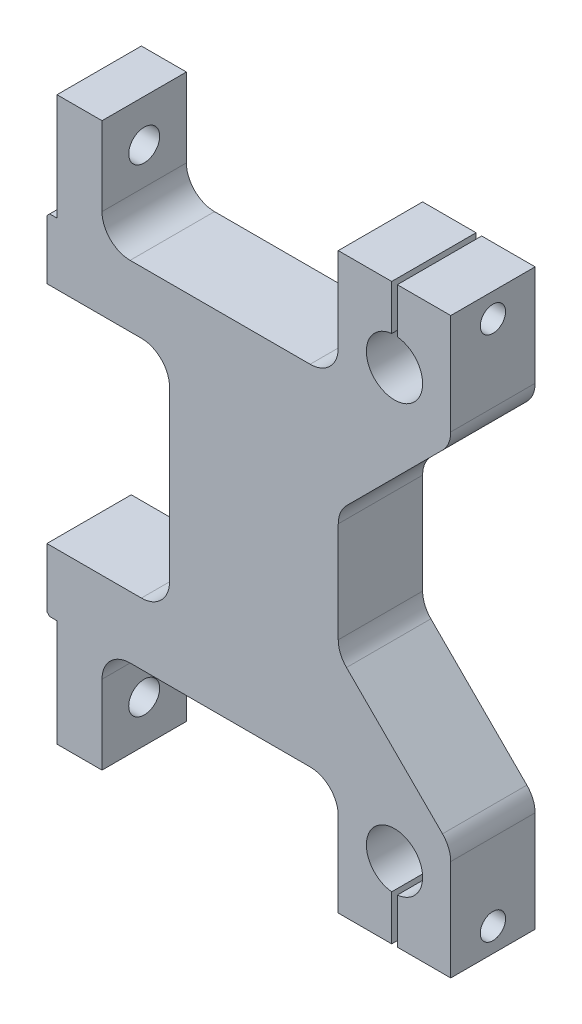
from build123d import *

# Parameters (mm, degrees)
BOSS_EXTRUDE1_DEPTH   = 40
SKETCH2_W             = 52
SKETCH2_H             = 20
CUT_EXTRUDE1_DEPTH    = 56
SKETCH3_R             = 5
CUT_EXTRUDE2_DEPTH    = 56
CHAMFER1_SIZE         = 20
SKETCH4_W             = 30
SKETCH4_H             = 11
BOSS_EXTRUDE2_DEPTH   = 15
SKETCH5_R             = 5
BOSS_EXTRUDE3_DEPTH   = 15
SKETCH6_W             = 45
SKETCH6_H             = 20
BOSS_EXTRUDE4_DEPTH   = 10
CUT_EXTRUDE3_REACH    = 134.714
SKETCH8_W             = 47.061475946
SKETCH8_H             = 40
SKETCH9_W             = 45
SKETCH9_H             = 19
BOSS_EXTRUDE5_DEPTH   = 8
SKETCH11_R            = 2.75
CUT_EXTRUDE4_DEPTH    = 37
SKETCH12_W            = 30
SKETCH12_H            = 100
CUT_EXTRUDE5_DEPTH    = 112
SKETCH13_W            = 0.2
SKETCH13_H            = 62
CUT_EXTRUDE6_DEPTH    = 112
CHAMFER2_SIZE         = 0.5
SKETCH14_W            = 1
SKETCH14_H            = 9.442903458
CUT_EXTRUDE7_DEPTH    = 29
SKETCH15_R            = 2.25
CUT_EXTRUDE8_DEPTH    = 9.5
M4_TAPPED_HOLE1_D     = 3.3
M4_TAPPED_HOLE1_DEPTH = 9.5
M4_TAPPED_HOLE2_D     = 3.3
M4_TAPPED_HOLE2_DEPTH = 9.5
FILLET1_R             = 5


with BuildPart() as part:
    # Sketch1 → Boss-Extrude1 (new body)
    with BuildSketch(Plane(origin=(0, 0, 0), x_dir=(1, 0, 0), z_dir=(0, 1, 0))):
        Polygon((0, 0), (72, 0), (72, 15), (10, 15), (10, 45), (0, 45), align=None)
    extrude(amount=BOSS_EXTRUDE1_DEPTH)

    # Sketch2 → Cut-Extrude1 (cut)
    with BuildSketch(Plane.XY):
        with Locations((26, 10)):
            Rectangle(SKETCH2_W, SKETCH2_H)
    extrude(amount=-CUT_EXTRUDE1_DEPTH, mode=Mode.SUBTRACT)

    # Sketch3 → Cut-Extrude2 (cut)
    with BuildSketch(Plane.XY):
        with Locations((62, 13)):
            Circle(SKETCH3_R)
    extrude(amount=-CUT_EXTRUDE2_DEPTH, mode=Mode.SUBTRACT)

    # Chamfer1
    chamfer1_edges = [part.edges().sort_by_distance(p)[0] for p in [
        (72, 40, -7.5),
    ]]
    chamfer(chamfer1_edges, length=CHAMFER1_SIZE)

    # Sketch4 → Boss-Extrude2 (add)
    with BuildSketch(Plane.XY):
        with Locations((37, 45.5)):
            Rectangle(SKETCH4_W, SKETCH4_H)
    extrude(amount=-BOSS_EXTRUDE2_DEPTH)

    # Sketch5 → Boss-Extrude3 (add)
    with BuildSketch(Plane.XY):
        Polygon((22, 51), (52, 51), (52, 62), (72, 82), (72, 102), (52, 102), (52, 82), (0, 82), (0, 62), (22, 62), align=None)
        with Locations((62, 89)):
            Circle(SKETCH5_R, mode=Mode.SUBTRACT)
    extrude(amount=-BOSS_EXTRUDE3_DEPTH)

    # Sketch6 → Boss-Extrude4 (add)
    with BuildSketch(Plane.ZY):
        with Locations((-22.5, 30)):
            Rectangle(SKETCH6_W, SKETCH6_H)
        with Locations((-22.5, 72)):
            Rectangle(SKETCH6_W, SKETCH6_H)
    extrude(amount=-BOSS_EXTRUDE4_DEPTH)

    # Cut-Extrude3: up to this face of the body (flat: up to its plane)
    cut_extrude3_end = Plane(part.part.faces().sort_by_distance((22, 51, -7.5))[0])
    # Sketch8 → Cut-Extrude3 (cut, up to the picked face)
    with BuildSketch(Plane.ZY, mode=Mode.PRIVATE) as cut_extrude3_sk1:
        with Locations((-21.469262027, 51)):
            Rectangle(SKETCH8_W, SKETCH8_H)
    cut_extrude3_tool1 = split(extrude(cut_extrude3_sk1.sketch, amount=-CUT_EXTRUDE3_REACH, mode=Mode.PRIVATE), bisect_by=cut_extrude3_end, keep=Keep.BOTH, mode=Mode.PRIVATE)
    add(cut_extrude3_tool1.solids().sort_by(Axis((0, 51, -21.469262), (1, 0, 0)))[0], mode=Mode.SUBTRACT)

    # Sketch9 → Boss-Extrude5 (add)
    with BuildSketch(Plane(origin=(10, 0, 0), x_dir=(0, 0, -1), z_dir=(1, 0, 0))):
        with Locations((22.5, 91.5)):
            Rectangle(SKETCH9_W, SKETCH9_H)
        with Locations((22.5, 10.5)):
            Rectangle(SKETCH9_W, SKETCH9_H)
    extrude(amount=-BOSS_EXTRUDE5_DEPTH)

    # Sketch11 → Cut-Extrude4 (cut)
    with BuildSketch(Plane(origin=(10, 0, 0), x_dir=(0, 0, -1), z_dir=(1, 0, 0))):
        with Locations((7.5, 93.5)):
            Circle(SKETCH11_R)
        with Locations(Location((7.5, 8.5, 0), (0, 0, 180))):
            Circle(SKETCH11_R)
    extrude(amount=-CUT_EXTRUDE4_DEPTH, mode=Mode.SUBTRACT)

    # Sketch12 → Cut-Extrude5 (cut)
    with BuildSketch(Plane(origin=(72, 0, 0), x_dir=(0, 0, -1), z_dir=(1, 0, 0))):
        with Locations((30, 51)):
            Rectangle(SKETCH12_W, SKETCH12_H)
    extrude(amount=-CUT_EXTRUDE5_DEPTH, mode=Mode.SUBTRACT)

    # Sketch13 → Cut-Extrude6 (cut)
    with BuildSketch(Plane.XY):
        with Locations((0.1, 51)):
            Rectangle(SKETCH13_W, SKETCH13_H)
    extrude(amount=-CUT_EXTRUDE6_DEPTH, mode=Mode.SUBTRACT)

    # Chamfer2
    chamfer2_edges = [part.edges().sort_by_distance(p)[0] for p in [
        (0.2, 20, -7.5),
        (0.2, 82, -7.5),
    ]]
    chamfer(chamfer2_edges, length=CHAMFER2_SIZE)

    # Sketch14 → Cut-Extrude7 (cut)
    with BuildSketch(Plane.XY):
        with Locations((62, 4.721451729)):
            Rectangle(SKETCH14_W, SKETCH14_H)
        with Locations((62, 97.278548271)):
            Rectangle(SKETCH14_W, SKETCH14_H)
    extrude(amount=-CUT_EXTRUDE7_DEPTH, mode=Mode.SUBTRACT)

    # Sketch15 → Cut-Extrude8 (cut)
    with BuildSketch(Plane(origin=(72, 0, 0), x_dir=(0, 0, -1), z_dir=(1, 0, 0))):
        with Locations((7.5, 97.75)):
            Circle(SKETCH15_R)
        with Locations((7.5, 4.25)):
            Circle(SKETCH15_R)
    extrude(amount=-CUT_EXTRUDE8_DEPTH, mode=Mode.SUBTRACT)

    # M4 Tapped Hole1
    with Locations(Plane(origin=(61.5, 97.75, -7.5), x_dir=(0, 0, 1), z_dir=(1, 0, 0))):
        with Locations((0, 0)):
            Hole(M4_TAPPED_HOLE1_D / 2, depth=M4_TAPPED_HOLE1_DEPTH)

    # M4 Tapped Hole2
    with Locations(Plane(origin=(61.5, 4.25, -7.5), x_dir=(0, 0, 1), z_dir=(1, 0, 0))):
        with Locations((0, 0)):
            Hole(M4_TAPPED_HOLE2_D / 2, depth=M4_TAPPED_HOLE2_DEPTH)

    # Fillet1
    fillet1_edges = [part.edges().sort_by_distance(p)[0] for p in [
        (72, 20, -7.5),
        (72, 82, -7.5),
        (52, 62, -7.5),
        (52, 40, -7.5),
        (52, 82, -7.5),
        (10, 82, -7.5),
        (22, 71, -7.5),
        (22, 31, -7.5),
        (10, 20, -7.5),
        (52, 20, -7.5),
    ]]
    fillet(fillet1_edges, radius=FILLET1_R)


solid = part.part
